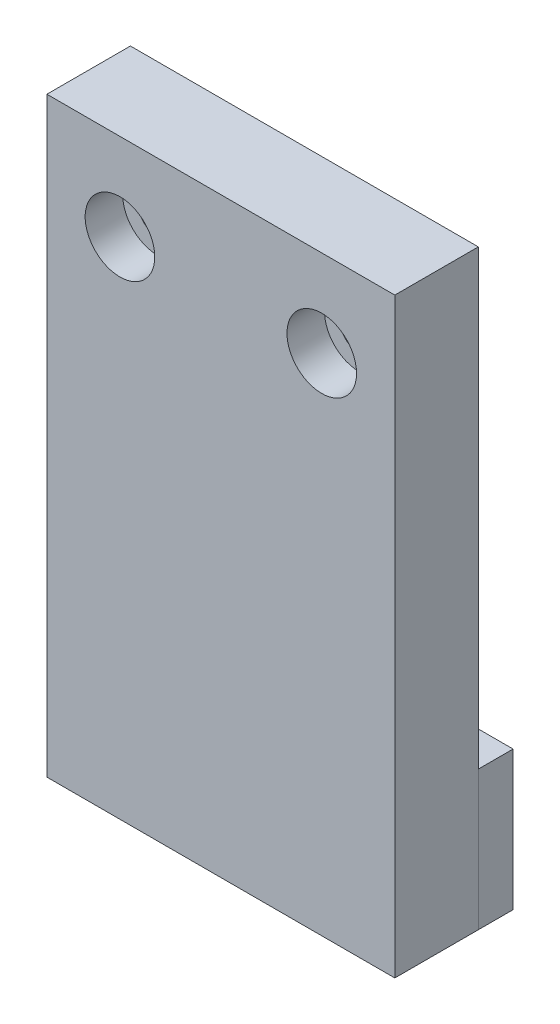
from build123d import *

# Parameters (mm, degrees)
SKETCH_1_W               = 50
SKETCH_1_H               = 85
EXTRUDE_1_DEPTH          = 6
SKETCH_2_W               = 50
SKETCH_2_H               = 20
EXTRUDE_2_DEPTH          = 5
HOLE_WIZARD_1_AT_2_COUNT = 2
HOLE_WIZARD_1_AT_2_PITCH = 29


with BuildPart() as part:
    # 草图1 → 凸台-拉伸1 (new, symmetric)
    with BuildSketch(Plane.XY):
        Rectangle(SKETCH_1_W, SKETCH_1_H)
    extrude(amount=EXTRUDE_1_DEPTH, both=True)

    # 草图3 → 打孔尺寸(%根据)内六角圆柱头螺钉的类型1 (revolve, cut)
    with BuildSketch(Plane(origin=(-14.5, 30, 6), x_dir=(0, -1, 0), z_dir=(1, 0, 0))):
        Polygon((0, 0), (0, 17), (2.75, 17), (2.75, 5.4), (5, 5.4), (5, 0), align=None)
    hole_wizard_1 = revolve(axis=Axis((-14.5, 30, 12.35), (0, 0, -1)), mode=Mode.SUBTRACT)

    # 打孔尺寸(%根据)内六角圆柱头螺钉的类型1 at 2: 打孔尺寸(%根据)内六角圆柱头螺钉的类型1 ×2
    with Locations(*[(i * HOLE_WIZARD_1_AT_2_PITCH, 0, 0) for i in range(1, HOLE_WIZARD_1_AT_2_COUNT)]):
        add(hole_wizard_1, mode=Mode.SUBTRACT)


with BuildPart() as body_2:
    # 草图2 → 凸台-拉伸2 (new body)
    with BuildSketch(Plane(origin=(0, 0, -6), x_dir=(-1, 0, 0), z_dir=(0, 0, -1))):
        with Locations((0, -32.5)):
            Rectangle(SKETCH_2_W, SKETCH_2_H)
    extrude(amount=EXTRUDE_2_DEPTH)


solid = Compound([part.part, body_2.part])
